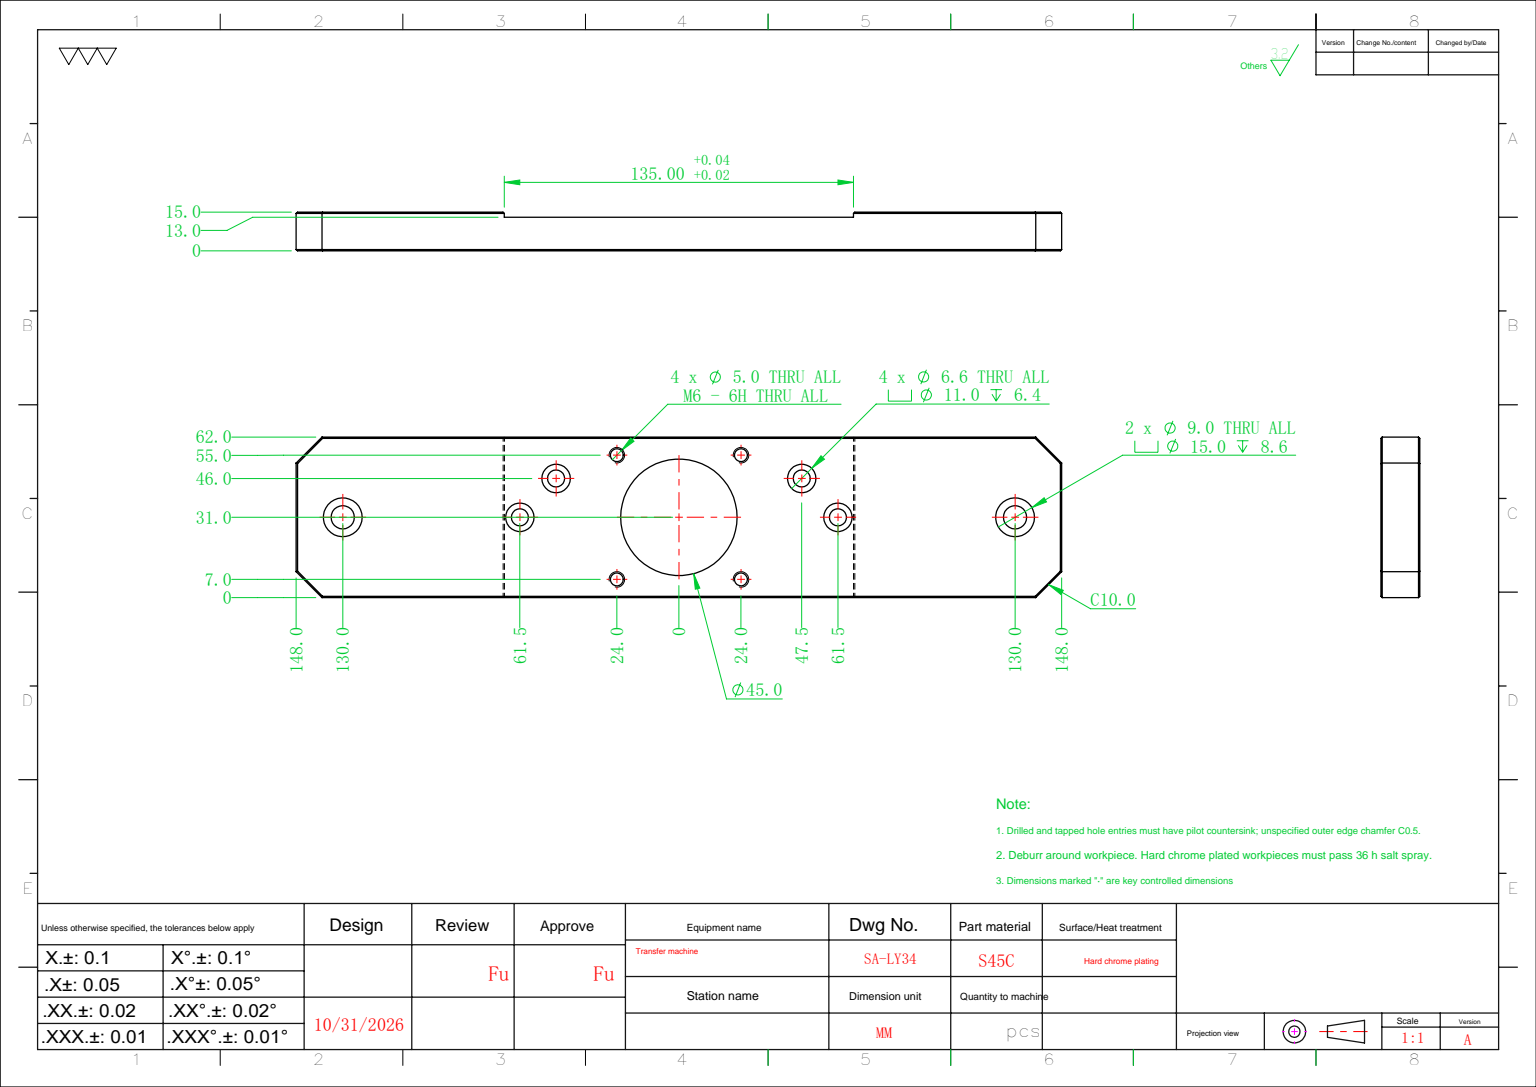
from build123d import *

# Parameters (mm, degrees)
SKETCH_1_W                     = 296
SKETCH_1_H                     = 62
EXTRUDE_1_DEPTH                = 15
CHAMFER_1_SIZE                 = 10
SKETCH_3_R                     = 22.5
CUT_EXTRUDE_2_DEPTH            = 152.95394039
HOLE_WIZARD_M6_1_D             = 5
SKETCH_6_W                     = 135
SKETCH_6_H                     = 2
CUT_EXTRUDE_3_DEPTH            = 162.161409773
HOLE_WIZARD_M6_1_2_D           = 6.6
HOLE_WIZARD_M6_1_2_CBORE_D     = 11
HOLE_WIZARD_M6_1_2_CBORE_DEPTH = 6.4
HOLE_WIZARD_M8_1_D             = 9
HOLE_WIZARD_M8_1_CBORE_D       = 15
HOLE_WIZARD_M8_1_CBORE_DEPTH   = 8.6
CHAMFER_2_SIZE                 = 0.5


with BuildPart() as part:
    # 草图1 → 凸台-拉伸1 (new body)
    with BuildSketch(Plane.XY):
        Rectangle(SKETCH_1_W, SKETCH_1_H)
    extrude(amount=EXTRUDE_1_DEPTH)

    # 倒角1
    chamfer_1_edges = [part.edges().sort_by_distance(p)[0] for p in [
        (148, -31, 7.5),
        (-148, -31, 7.5),
        (-148, 31, 7.5),
        (148, 31, 7.5),
    ]]
    chamfer(chamfer_1_edges, length=CHAMFER_1_SIZE)

    # 草图3 → 切除-拉伸2 (cut, through all)
    with BuildSketch(Plane(origin=(0, 0, 0), x_dir=(-1, 0, 0), z_dir=(0, 0, -1))):
        Circle(SKETCH_3_R)
    extrude(amount=-CUT_EXTRUDE_2_DEPTH, mode=Mode.SUBTRACT)

    # Hole Wizard M6 _1 (through all)
    with Locations(Plane.XY.offset(15)):
        with Locations((-24, 24), (24, 24), (24, -24), (-24, -24)):
            Hole(HOLE_WIZARD_M6_1_D / 2)

    # 草图6 → 切除-拉伸3 (cut, through all)
    with BuildSketch(Plane.XZ.offset(31)):
        with Locations((0, 1)):
            Rectangle(SKETCH_6_W, SKETCH_6_H)
    extrude(amount=-CUT_EXTRUDE_3_DEPTH, mode=Mode.SUBTRACT)

    # Hole Wizard M6 _1 2 (through all)
    with Locations(Plane.XY.offset(15)):
        with Locations((-47.5, 15), (-61.5, 0), (47.5, 15), (61.5, 0)):
            CounterBoreHole(HOLE_WIZARD_M6_1_2_D / 2, HOLE_WIZARD_M6_1_2_CBORE_D / 2, HOLE_WIZARD_M6_1_2_CBORE_DEPTH)

    # M8 六角凹头螺钉的柱形沉头孔1 (through all)
    with Locations(Plane(origin=(0, 0, 15), x_dir=(-1, 0, 0), z_dir=(0, 0, 1))):
        with Locations((130, 0), (-130, 0)):
            CounterBoreHole(HOLE_WIZARD_M8_1_D / 2, HOLE_WIZARD_M8_1_CBORE_D / 2, HOLE_WIZARD_M8_1_CBORE_DEPTH)

    # 倒角2
    chamfer_2_edges = [part.edges().sort_by_distance(p)[0] for p in [
        (102.75, 31, 0),
        (0, 31, 15),
        (148, 0, 0),
        (-102.75, -31, 0),
        (-148, 0, 0),
        (-143, -26, 0),
        (-143, 26, 0),
        (143, -26, 0),
        (143, 26, 0),
        (148, 0, 15),
        (-148, 0, 15),
        (0, -31, 15),
        (-143, -26, 15),
        (-143, 26, 15),
        (143, -26, 15),
        (143, 26, 15),
        (-102.75, 31, 0),
        (102.75, -31, 0),
        (67.5, 0, 0),
        (-67.5, 0, 0),
    ]]
    chamfer(chamfer_2_edges, length=CHAMFER_2_SIZE)


solid = part.part
